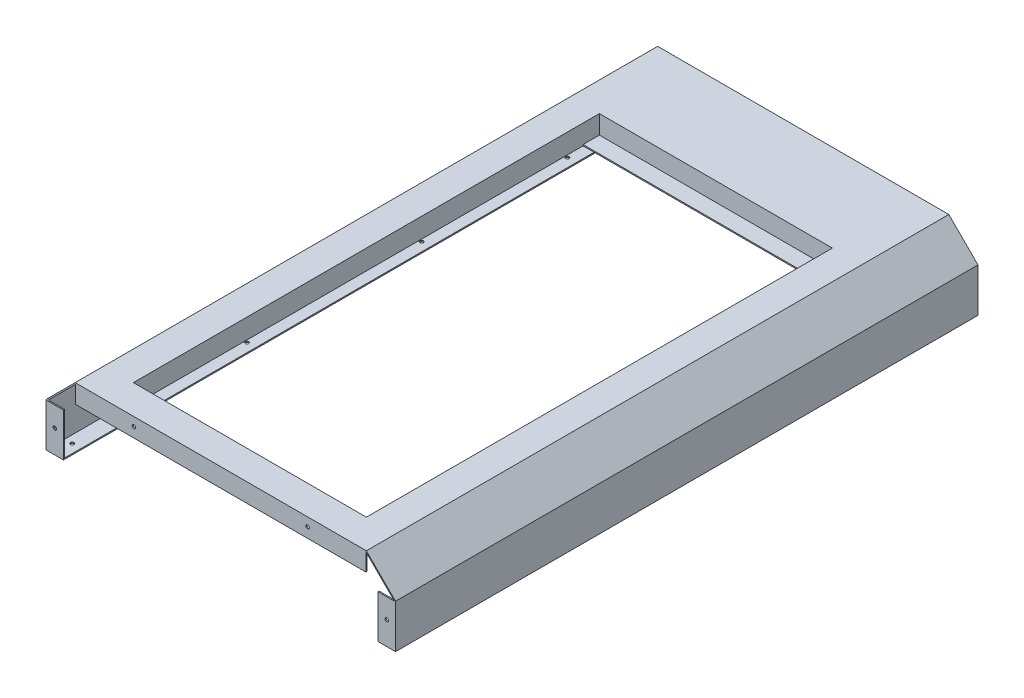
SolidWorks part; units mm, degrees
ref_plane "前视" through (0, 0, 0) normal (0, 0, 1) x (1, 0, 0)
ref_plane "上视" through (0, 0, 0) normal (0, 1, 0) x (1, 0, 0)
ref_plane "右视" through (0, 0, 0) normal (1, 0, 0) x (0, 0, -1)
sketch "草图1" plane through (0, 0, 0) normal (0, 0, 1) x (1, 0, 0)
  line L0 (0, 700) -> (50, 750)
  line L1 (0, 0) -> (600, 0)
  line L2 (0, 0) -> (0, 700)
  line L3 (50, 750) -> (550, 750)
  line L4 (600, 0) -> (600, 700)
  line L5 (550, 750) -> (600, 700)
  point P1 (600, 750)
  point P3 (0, 750)
  dimension "D1" = 600
  dimension "D2" = 750
extrude "凸台-拉伸1" add sketch "草图1" along normal blind 1000
shell "抽壳1" thickness 2
sketch "草图3" plane through (0, 750, 0) normal (0, 1, 0) x (1, 0, 0)
  line L0 (0, -1000) -> (0, 0) construction
  line L1 (100, -150) -> (500, -150)
  line L2 (100, -150) -> (100, -950)
  line L3 (100, -950) -> (500, -950)
  line L4 (500, -150) -> (500, -950)
  line L5 (550, 0) -> (50, 0) construction
  dimension "D1" = 100
  dimension "D2" = 150
  dimension "D3" = 800
  dimension "D4" = 400
extrude "切除-拉伸1" cut sketch "草图3" against normal blind 30
sketch "草图4" plane through (0, 750, 0) normal (0, 1, 0) x (1, 0, 0)
  line L0 (98, -148) -> (502, -148)
  line L1 (100, -150) -> (500, -150)
  line L2 (100, -150) -> (100, -950)
  line L3 (100, -950) -> (500, -950)
  line L4 (500, -150) -> (500, -950)
  line L5 (502, -148) -> (502, -952)
  line L6 (98, -952) -> (502, -952)
  line L7 (98, -148) -> (98, -952)
  dimension "D1" = 2
extrude "凸台-拉伸2" add sketch "草图4" against normal blind 34
sketch "草图5" plane through (0, 716, 0) normal (0, -1, 0) x (1, 0, 0)
  line L0 (128, 178) -> (472, 178)
  line L1 (100, 150) -> (500, 150)
  line L2 (100, 150) -> (100, 178)
  line L3 (100, 950) -> (500, 950)
  line L4 (500, 150) -> (500, 950)
  line L5 (472, 178) -> (472, 922)
  line L6 (128, 922) -> (472, 922)
  line L8 (128, 178) -> (100, 178)
  line L9 (128, 922) -> (100, 922)
  line L10 (100, 922) -> (100, 950)
  line L12 (100, 150) -> (100, 950) construction
  line L18 (128, 178) -> (128, 922) construction
  point P0 (178, 148)
  point P1 (582, 802)
  point P2 (178, 802)
  point P3 (582, 148)
  dimension "D1" = 28
extrude "凸台-拉伸3" add sketch "草图5" against normal blind 2
sketch "草图6" plane through (0, 0, 0) normal (0, 0, -1) x (-1, 0, 0)
  line L0 (-600, 0) -> (-600, 700) construction
  line L1 (0, 0) -> (-600, 0)
  line L2 (0, 0) -> (0, 200)
  line L3 (0, 200) -> (-600, 200)
  line L4 (-600, 0) -> (-600, 200)
  dimension "D1" = 200
extrude "切除-拉伸2" cut sketch "草图6" against normal blind 1044
sketch "草图10" plane through (0, 0, 0) normal (0, 0, -1) x (-1, 0, 0)
  line L0 (-600, 200) -> (-600, 700) construction
  line L1 (0, 200) -> (-600, 200)
  line L2 (0, 200) -> (0, 625)
  line L3 (0, 625) -> (-600, 625)
  line L4 (-600, 200) -> (-600, 625)
  dimension "D1" = 425
extrude "切除-拉伸4" cut sketch "草图10" against normal blind 1005
sketch "草图11" plane through (0, 625, 0) normal (0, -1, 0) x (1, 0, 0)
  line L0 (549.1716, 1000) -> (50.8284, 1000) construction
  line L1 (2, 2) -> (30, 2)
  line L2 (2, 2) -> (2, 1000)
  line L3 (2, 1000) -> (30, 1000)
  line L4 (30, 2) -> (30, 1000)
  line L6 (598, 2) -> (570, 2)
  line L7 (598, 2) -> (598, 1000)
  line L8 (598, 1000) -> (570, 1000)
  line L9 (570, 2) -> (570, 1000)
  dimension "D1" = 28
  dimension "D2" = 28
extrude "凸台-拉伸5" add sketch "草图11" against normal blind 2
sketch "草图12" plane through (0, 0, 1000) normal (0, 0, 1) x (1, 0, 0)
  line L0 (549.1716, 748) -> (549.1716, 718)
  line L1 (2, 699.1716) -> (30, 699.1716)
  line L2 (2, 699.1716) -> (2, 627)
  line L3 (2, 627) -> (30, 627)
  line L4 (30, 699.1716) -> (30, 627)
  line L5 (598, 699.1716) -> (570, 699.1716)
  line L6 (598, 699.1716) -> (598, 627)
  line L7 (598, 627) -> (570, 627)
  line L8 (570, 699.1716) -> (570, 627)
  line L9 (50.8284, 748) -> (549.1716, 748)
  line L10 (50.8284, 748) -> (50.8284, 718)
  line L11 (50.8284, 718) -> (549.1716, 718)
  dimension "D1" = 30
extrude "凸台-拉伸6" add sketch "草图12" against normal blind 2
sketch "草图13" plane through (0, 0, 1000) normal (0, 0, 1) x (1, 0, 0)
  line L0 (600, 625) -> (600, 700) construction
  line L1 (570, 625) -> (600, 625) construction
  line L2 (300, 625) -> (300, 818.6104) construction
  line L3 (30, 625) -> (570, 625) construction
  circle A0 centre (585, 665) radius 3
  circle A1 centre (15, 665) radius 3
  dimension "D1" = 6
  dimension "D2" = 15
  dimension "D3" = 40
extrude "切除-拉伸5" cut sketch "草图13" against normal blind 1280
sketch "草图14" plane through (0, 625, 0) normal (0, -1, 0) x (1, 0, 0)
  line L0 (15, 970) -> (15, -54.6994) construction
  line L1 (0, 1000) -> (0, 0) construction
  line L2 (0, 1000) -> (30, 1000) construction
  line L3 (300, 998) -> (300, 492.0189) construction
  line L4 (50.8284, 998) -> (549.1716, 998) construction
  circle A0 centre (15, 970) radius 3
  circle A1 centre (15, 670) radius 3
  circle A2 centre (585, 120) radius 3
  circle A3 centre (15, 370) radius 3
  circle A4 centre (585, 370) radius 3
  circle A5 centre (15, 120) radius 3
  circle A6 centre (585, 670) radius 3
  circle A7 centre (585, 970) radius 3
  dimension "D3" = 6
  dimension "D4" = 6
  dimension "D5" = 300
  dimension "D6" = 6
  dimension "D8" = 300
  dimension "D9" = 250
  dimension "D10" = 6
  dimension "D1" = 15
  dimension "D2" = 30
extrude "切除-拉伸6" cut sketch "草图14" against normal blind 10
sketch "草图15" plane through (0, 0, 1000) normal (0, 0, 1) x (1, 0, 0)
  line L0 (150.8284, 735) -> (711.3256, 735) construction
  line L1 (550, 750) -> (50, 750) construction
  line L2 (50.8284, 748) -> (50.8284, 718) construction
  line L4 (549.1716, 718) -> (549.1716, 748) construction
  circle A0 centre (150.8284, 735) radius 3
  circle A1 centre (449.1716, 735) radius 3
  dimension "D1" = 6
  dimension "D3" = 6
  dimension "D4" = 100
  dimension "D5" = 100
  dimension "D2" = 15
extrude "切除-拉伸7" cut sketch "草图15" against normal blind 28
sketch "草图16" plane through (0, 0, 0) normal (0, 0, -1) x (-1, 0, 0)
  line L0 (-550, 750) -> (-50, 750) construction
  circle A0 centre (-450, 735) radius 3
  circle A1 centre (-150, 734.7261) radius 3
  dimension "D1" = 6
  dimension "D2" = 15
  dimension "D3" = 100
  dimension "D4" = 6
  dimension "D5" = 100
extrude "切除-拉伸8" cut sketch "草图16" against normal blind 10
